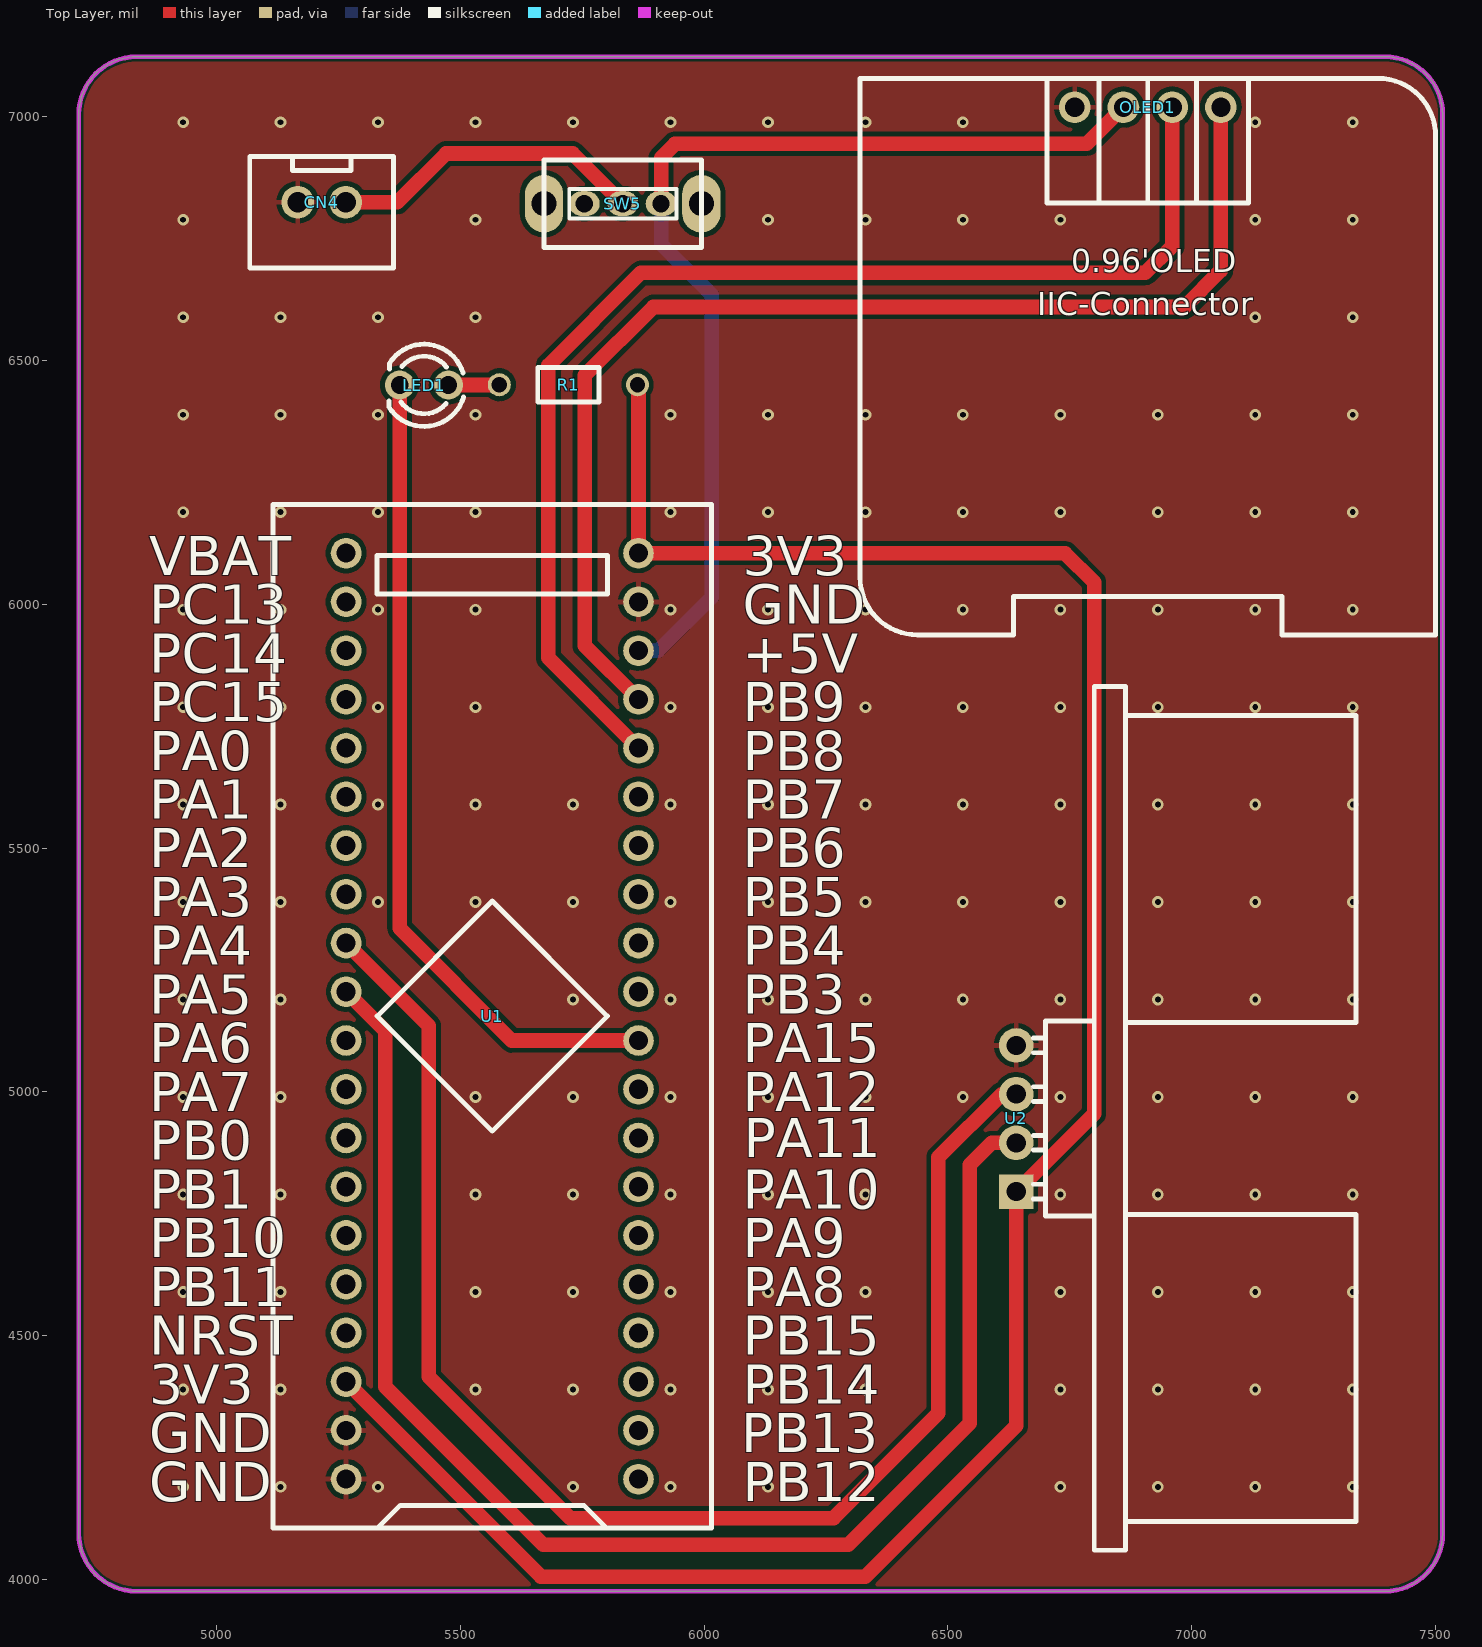
[diagram p0: Top Layer view]
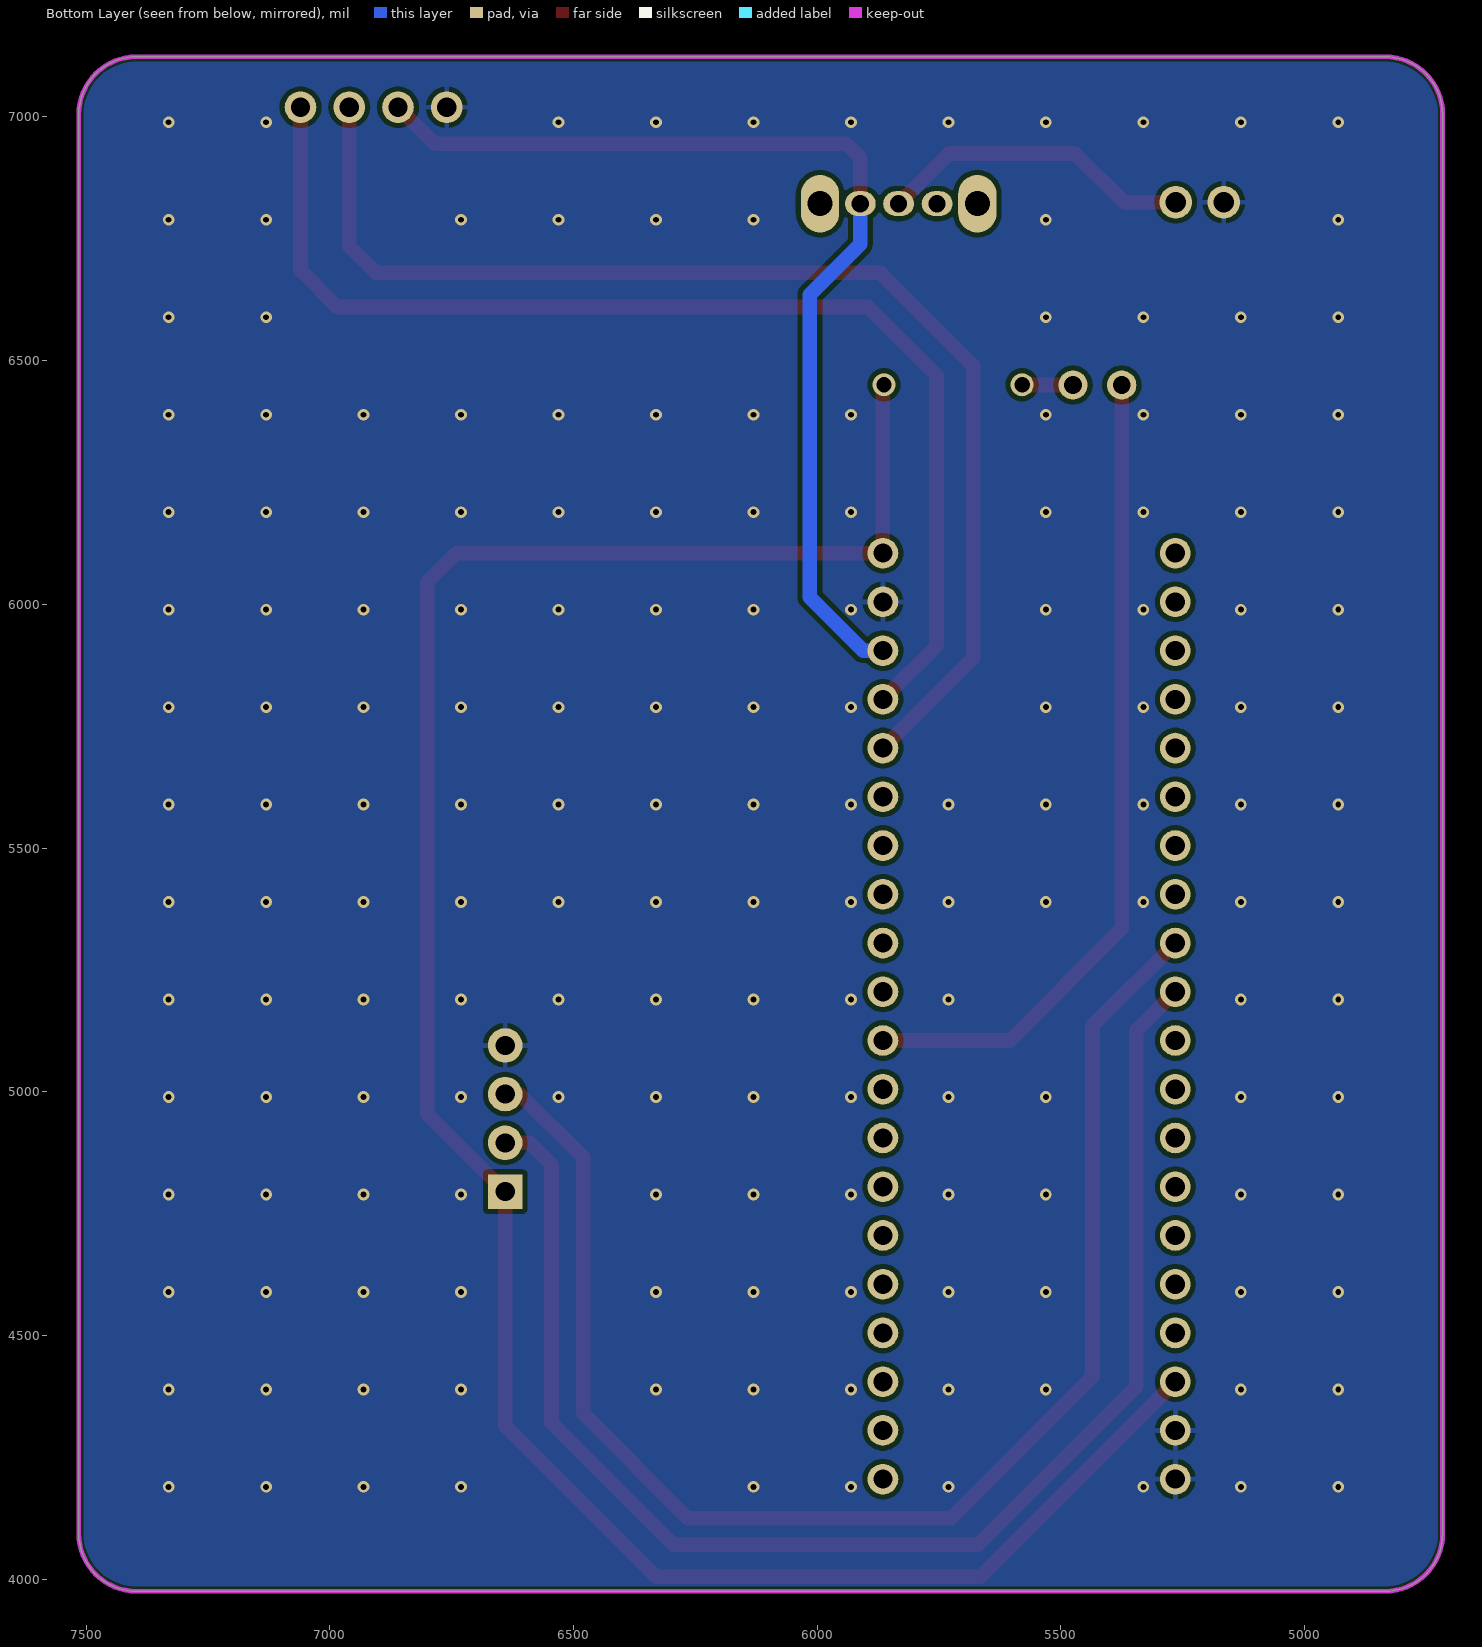
[diagram p1: Bottom Layer view, seen from below]
# Altium PCB MISC89090.pcbdoc
Units mil, origin at the board's own origin, x right, y up, seen from the top; angles counter-clockwise.
Board outline 2798.5 x 3148.5 mil, 2 copper layers (Top Layer, Bottom Layer), stack 62.206 mil thick; 7 components, 39 nets, 59 pads, 165 vias.

## Layer stack, top to bottom
Top Solder Mask Layer: solder mask 0.394, Dk 3.3
Top Layer: signal copper 1.379
Dielectric1: surface 59.449, FR4, Dk 4.5
Bottom Layer: signal copper 1.378
Bottom Solder Mask Layer: solder mask 0.394, Dk 3.3

## Board outline
4834.61,7123.5 ccw(c4834.61,7005.39) 4716.5,7005.39 4716.5,4093.11 ccw(c4834.61,4093.11) 4834.61,3975 7396.89,3975 ccw(c7396.89,4093.11) 7515,4093.11 7515,7005.39 ccw(c7396.89,7005.39) 7396.89,7123.5 4834.61,7123.5

## Design rules (kind name [scope] priority, off if disabled: settings)
BoardOutlineClearance copperThickness2oz_1 [All] p2 off: genericclearance=7.99 ignorepadtopadclearanceinfootprint=FALSE except(0: Arc-SplitContinuation Track-SplitContinuation SMDPad-SplitContinuation THPad-SplitContinuation Via-SplitContinuation Fill-SplitContinuation Region-SplitContinuation Poly-SplitContinuation Text-SplitContinuation Hole-SplitContinuation; 5.98: Arc-CutoutEdge Track-CutoutEdge SMDPad-CutoutEdge THPad-CutoutEdge Via-CutoutEdge Text-CutoutEdge; 6.9: Hole-OutlineEdge Hole-CutoutEdge; 10: Poly-OutlineEdge Poly-CutoutEdge; 11.81: Arc-OutlineEdge Track-OutlineEdge SMDPad-OutlineEdge THPad-OutlineEdge Via-OutlineEdge Fill-OutlineEdge Region-OutlineEdge Text-OutlineEdge Fill-CutoutEdge Region-CutoutEdge)
BoardOutlineClearance Plane_innerPlane_1 [All] p4 off: genericclearance=4.02 ignorepadtopadclearanceinfootprint=FALSE except(0: Arc-SplitContinuation Track-SplitContinuation SMDPad-SplitContinuation THPad-SplitContinuation Via-SplitContinuation Fill-SplitContinuation Region-SplitContinuation Poly-SplitContinuation Text-SplitContinuation Hole-SplitContinuation; 5.98: Arc-CutoutEdge Track-CutoutEdge SMDPad-CutoutEdge THPad-CutoutEdge Via-CutoutEdge Text-CutoutEdge; 6.9: Hole-OutlineEdge Hole-CutoutEdge; 10: Poly-OutlineEdge Poly-CutoutEdge; 11.81: Arc-OutlineEdge Track-OutlineEdge SMDPad-OutlineEdge THPad-OutlineEdge Via-OutlineEdge Fill-OutlineEdge Region-OutlineEdge Text-OutlineEdge Fill-CutoutEdge Region-CutoutEdge)
BoardOutlineClearance Copper_copperRegion_1 [All] p6 off: genericclearance=4.02 ignorepadtopadclearanceinfootprint=FALSE except(0: Arc-SplitContinuation Track-SplitContinuation SMDPad-SplitContinuation THPad-SplitContinuation Via-SplitContinuation Fill-SplitContinuation Region-SplitContinuation Poly-SplitContinuation Text-SplitContinuation Hole-SplitContinuation; 5.98: Arc-CutoutEdge Track-CutoutEdge SMDPad-CutoutEdge THPad-CutoutEdge Via-CutoutEdge Text-CutoutEdge; 6.9: Hole-OutlineEdge Hole-CutoutEdge; 10: Poly-OutlineEdge Poly-CutoutEdge; 11.81: Arc-OutlineEdge Track-OutlineEdge SMDPad-OutlineEdge THPad-OutlineEdge Via-OutlineEdge Fill-OutlineEdge Region-OutlineEdge Text-OutlineEdge Fill-CutoutEdge Region-CutoutEdge)
BoardOutlineClearance copperThickness1oz_1 [All] p8: genericclearance=4.02 ignorepadtopadclearanceinfootprint=FALSE except(0: Arc-SplitContinuation Track-SplitContinuation SMDPad-SplitContinuation THPad-SplitContinuation Via-SplitContinuation Fill-SplitContinuation Region-SplitContinuation Poly-SplitContinuation Text-SplitContinuation Hole-SplitContinuation; 5.98: Arc-CutoutEdge Track-CutoutEdge SMDPad-CutoutEdge THPad-CutoutEdge Via-CutoutEdge Text-CutoutEdge; 6.9: Hole-OutlineEdge Hole-CutoutEdge; 10: Poly-OutlineEdge Poly-CutoutEdge; 11.81: Arc-OutlineEdge Track-OutlineEdge SMDPad-OutlineEdge THPad-OutlineEdge Via-OutlineEdge Fill-OutlineEdge Region-OutlineEdge Text-OutlineEdge Fill-CutoutEdge Region-CutoutEdge)
Clearance copperThickness2oz [All] p1 off: gap=7.99 ignorepadtopadclearanceinfootprint=FALSE except(5.98: SMDPad-Track SMDPad-SMDPad THPad-Track SMDPad-THPad THPad-THPad Track-Via SMDPad-Via THPad-Via Via-Via Fill-SMDPad Region-SMDPad Fill-THPad Region-THPad Fill-Via Region-Via Fill-Fill Fill-Region Region-Region Arc-Track Arc-SMDPad Arc-THPad Arc-Via Fill-Arc Region-Arc Arc-Arc Text-Track SMDPad-Text Text-THPad Text-Via Fill-Text Region-Text Arc-Text Text-Text; 6.9: Hole-Track Hole-SMDPad Hole-THPad Hole-Via Fill-Hole Region-Hole Hole-Arc Hole-Text; 10: Poly-Track Poly-SMDPad Poly-THPad Poly-Via Poly-Fill Poly-Region Poly-Poly Poly-Arc Poly-Text Poly-Hole; 11.81: Fill-Track Region-Track)
Clearance Plane_innerPlane [All] p3 off: gap=4.02 ignorepadtopadclearanceinfootprint=FALSE except(5.98: SMDPad-Track SMDPad-SMDPad THPad-Track SMDPad-THPad THPad-THPad Track-Via SMDPad-Via THPad-Via Via-Via Fill-SMDPad Region-SMDPad Fill-THPad Region-THPad Fill-Via Region-Via Fill-Fill Fill-Region Region-Region Arc-Track Arc-SMDPad Arc-THPad Arc-Via Fill-Arc Region-Arc Arc-Arc Text-Track SMDPad-Text Text-THPad Text-Via Fill-Text Region-Text Arc-Text Text-Text; 6.9: Hole-Track Hole-SMDPad Hole-THPad Hole-Via Fill-Hole Region-Hole Hole-Arc Hole-Text; 10: Poly-Track Poly-SMDPad Poly-THPad Poly-Via Poly-Fill Poly-Region Poly-Poly Poly-Arc Poly-Text Poly-Hole; 11.81: Fill-Track Region-Track)
Clearance Copper_copperRegion [All] p5 off: gap=4.02 ignorepadtopadclearanceinfootprint=FALSE except(5.98: SMDPad-Track SMDPad-SMDPad THPad-Track SMDPad-THPad THPad-THPad Track-Via SMDPad-Via THPad-Via Via-Via Fill-SMDPad Region-SMDPad Fill-THPad Region-THPad Fill-Via Region-Via Fill-Fill Fill-Region Region-Region Arc-Track Arc-SMDPad Arc-THPad Arc-Via Fill-Arc Region-Arc Arc-Arc Text-Track SMDPad-Text Text-THPad Text-Via Fill-Text Region-Text Arc-Text Text-Text; 6.9: Hole-Track Hole-SMDPad Hole-THPad Hole-Via Fill-Hole Region-Hole Hole-Arc Hole-Text; 10: Poly-Track Poly-SMDPad Poly-THPad Poly-Via Poly-Fill Poly-Region Poly-Poly Poly-Arc Poly-Text Poly-Hole; 11.81: Fill-Track Region-Track)
Clearance copperThickness1oz [All] p7: gap=4.02 ignorepadtopadclearanceinfootprint=FALSE except(5.98: SMDPad-Track SMDPad-SMDPad THPad-Track SMDPad-THPad THPad-THPad Track-Via SMDPad-Via THPad-Via Via-Via Fill-SMDPad Region-SMDPad Fill-THPad Region-THPad Fill-Via Region-Via Fill-Fill Fill-Region Region-Region Arc-Track Arc-SMDPad Arc-THPad Arc-Via Fill-Arc Region-Arc Arc-Arc Text-Track SMDPad-Text Text-THPad Text-Via Fill-Text Region-Text Arc-Text Text-Text; 6.9: Hole-Track Hole-SMDPad Hole-THPad Hole-Via Fill-Hole Region-Hole Hole-Arc Hole-Text; 10: Poly-Track Poly-SMDPad Poly-THPad Poly-Via Poly-Fill Poly-Region Poly-Poly Poly-Arc Poly-Text Poly-Hole; 11.81: Fill-Track Region-Track)
DiffPairsRouting differentialPair [All] p1: maxlimit=6 minlimit=6 mostfreqgap=6 toplayer_minwidth=5 toplayer_prefwidth=10 toplayer_maxwidth=100 toplayer_mingap=6 toplayer_prefgap=6 toplayer_maxgap=6 bottomlayer_minwidth=5 bottomlayer_prefwidth=10 bottomlayer_maxwidth=100 bottomlayer_mingap=6 bottomlayer_prefgap=6 bottomlayer_maxgap=6 maxuncoupledlength=10
HoleToHoleClearance otherClearance [All] p1: gap=11.81 allowstackedmicrovias=TRUE
Length netLength [All] p1: minlimit=0 maxlimit=0
PasteMaskExpansion pasteMaskExpansion [All] p1: expansion=0
PlaneConnect innerPlane [All] p1: planeconnectstyle=Relief reliefexpansion=20 reliefentries=4 reliefconductorwidth=10 reliefairgap=10
PolygonConnect copperRegion [All] p1: connectstyle=Relief reliefconductorwidth=10 reliefentries=4 polygonreliefangle="90 Angle" airgapwidth=10 via.connectstyle=Relief via.reliefconductorwidth=10 via.reliefentries=4 via.polygonreliefangle="90 Angle" via.airgapwidth=10
RoutingVias viaSize [All] p1: holewidth=12.01 width=24.02 viastyle="Through Hole" minholewidth=11.81 minwidth=19.68 maxholewidth=248.03 maxwidth=393.7
SolderMaskExpansion solderMaskExpansion [IsVia] p1: expansion=-1000 istentingtop=TRUE
SolderMaskExpansion solderMaskExpansion [All] p2: expansion=2 istentingtop=FALSE
Width copperThickness2oz_2 [All] p1 off: maxlimit=100 minlimit=8 preferedwidth=10
Width copperThickness1oz_2 [All] p2: maxlimit=100 minlimit=5 preferedwidth=10

## Components (designator, comment, footprint, x,y, rotation, side; value= is the part's Value field where it differs from the comment)
CN4 "XH2.54*2P_Through-hole" CONN-TH_2P-P2.50-XH2.54-2P 5215,6825 r0 top
LED1 "" LED_TH-3mm 5425,6450 r180 top
OLED1 "" 0.96OLED_4P 6910,7020 r0 top
R1 "220Ω" Res_1/8W 5721.15,6448.05 r0 top
SW5 "" 拨动开关 5837.9,6822.05 r180 top
U1 "STM32F103C8T6-Card" CONN-TH_L53.3-W22.9_STM32F103C8T6-CARD 5565,5155 r90 top
U2 "HC-SR04" TH_HC-SR04V 6640,4945 r90 top

## Footprints (in the part's own frame and the unit in brackets; to place one, negate y for a bottom-side part, rotate by r counter-clockwise, add the part's x,y. Pads: shape width x height; smd on the part's side, far side on the other; paste and mask are expansions set on the pad)
0.96OLED_4P [mm]
  round 1.65 hole 1 copper offset 0,0: 1(-3.81,-0.001) 2(-1.27,0.002) 3(1.27,0.002) 4(3.81,0.002)
  silkscreen extent -15,-27.5 15,1.5
CONN-TH_2P-P2.50-XH2.54-2P [mm]
  round 1.7 hole 1.05 paste+0 mask+0.05: 1(1.25,0) 2(-1.25,0)
  silkscreen extent -3.75,-3.42 3.75,2.37
CONN-TH_L53.3-W22.9_STM32F103C8T6-CARD [mm]
  round 1.6 hole 1: 1(-24.13,-7.62) 2(-21.59,-7.62) 3(-19.05,-7.62) 4(-16.51,-7.62) 5(-13.97,-7.62) 6(-11.43,-7.62) 7(-8.89,-7.62) 8(-6.35,-7.62) 9(-3.81,-7.62) 10(-1.27,-7.62) 11(1.27,-7.62) 12(3.81,-7.62) 13(6.35,-7.62) 14(8.89,-7.62) 15(11.43,-7.62) 16(13.97,-7.62) 17(16.51,-7.62) 18(19.05,-7.62) 19(21.59,-7.62) 20(24.13,-7.62) 21(24.13,7.62) 22(21.59,7.62) 23(19.05,7.62) 24(16.51,7.62) 25(13.97,7.62) 26(11.43,7.62) 27(8.89,7.62) 28(6.35,7.62) 29(3.81,7.62) 30(1.27,7.62) 31(-1.27,7.62) 32(-3.81,7.62) 33(-6.35,7.62) 34(-8.89,7.62) 35(-11.43,7.62) 36(-13.97,7.62) 37(-16.51,7.62) 38(-19.05,7.62) 39(-21.59,7.62) 40(-24.13,7.62)
  silkscreen extent -26.67,-11.43 26.67,11.43
LED_TH-3mm [mil]
  round 60 hole 36 paste+0 mask+2: 1(-50,0) 2(50,0)
  silkscreen extent -81,-84 72,85
Res_1/8W [mil]
  round 47.2 hole 31.5 paste+0 mask+2: 1(-141.7,2.48) 2(141.7,2.48)
  silkscreen extent -63,-33 63,38
TH_HC-SR04V [mm]
  rect 1.8x1.8 hole 1.001: 1(-3.81,0)
  round 1.8 hole 1.001: 2(-1.27,0) 3(1.27,0) 4(3.81,0)
  silkscreen extent -22.5,-17.7 22.5,-0.89
拨动开关 [mil]
  oval 63x51.2 hole 35.4 paste+0 mask+2: 1(-73.4,0) 2(5,0) 3(84,0)
  oval 78.7x118.1 hole 51.2 paste+0 mask+2: 4(166.7,0) 5(-156.1,0)
  silkscreen extent -156,-90 167,90

## Via types
v1: diameter 24.02, hole 12, Top Layer to Bottom Layer, 165 vias

## Nets (pads, with @x,y where several pads share a name; then routed paths per layer and width w, separated by ;. In a path a pad name is that pad's centre, name@x,y a point inside that pad or via, vN(x,y) a via of type N, cw(c..) or ccw(c..) an arc to the next point about the centre after c; other vN are vias at no path point)
$1N17118: CN4.1 SW5.2 | length 652.7
  Top Layer w30: CN4.1 5370,6825 5470,6925 5729.95,6925 SW5.2
$1N17142: LED1.1 R1.1 | length 104.7
  Top Layer w30: LED1.1 5578.92,6450 R1.1
+5V: OLED1.2 SW5.1 U1.18 | length 2131.5
  Top Layer w30: SW5.1 5911.3,6916.3 5940,6945 6784.95,6945 OLED1.2@6860,7020.05
  Bottom Layer w30: U1.18 5905,5905 6015,6015 6015,6635 5911.3,6738.7 SW5.1
GND: CN4.2 OLED1.1 U1.19 U1.39 U1.40 U2.4
  other v1: 4930.6,4189.1 5130.6,4189.1 5330.6,4189.1 5730.6,4189.1 5930.6,4189.1 6130.6,4189.1 6730.6,4189.1 6930.6,4189.1 7130.6,4189.1 7330.6,4189.1 4930.6,4389.1 5130.6,4389.1 5530.6,4389.1 5730.6,4389.1 5930.6,4389.1 6130.6,4389.1 6330.6,4389.1 6730.6,4389.1 6930.6,4389.1 7130.6,4389.1 7330.6,4389.1 4930.6,4589.1 5130.6,4589.1 5530.6,4589.1 5730.6,4589.1 5930.6,4589.1 6130.6,4589.1 6330.6,4589.1 6730.6,4589.1 6930.6,4589.1 7130.6,4589.1 7330.6,4589.1 4930.6,4789.1 5130.6,4789.1 5530.6,4789.1 5730.6,4789.1 5930.6,4789.1 6130.6,4789.1 6330.6,4789.1 6730.6,4789.1 6930.6,4789.1 7130.6,4789.1 7330.6,4789.1 4930.6,4989.1 5130.6,4989.1 5530.6,4989.1 5730.6,4989.1 5930.6,4989.1 6130.6,4989.1 6330.6,4989.1 6530.6,4989.1 6730.6,4989.1 6930.6,4989.1 7130.6,4989.1 7330.6,4989.1 4930.6,5189.1 5130.6,5189.1 5730.6,5189.1 5930.6,5189.1 6130.6,5189.1 6330.6,5189.1 6530.6,5189.1 6730.6,5189.1 6930.6,5189.1 7130.6,5189.1 7330.6,5189.1 4930.6,5389.1 5130.6,5389.1 5330.6,5389.1 5530.6,5389.1 5730.6,5389.1 5930.6,5389.1 6130.6,5389.1 6330.6,5389.1 6530.6,5389.1 6730.6,5389.1 6930.6,5389.1 7130.6,5389.1 7330.6,5389.1 4930.6,5589.1 5130.6,5589.1 5330.6,5589.1 5530.6,5589.1 5730.6,5589.1 5930.6,5589.1 6130.6,5589.1 6330.6,5589.1 6530.6,5589.1 6730.6,5589.1 6930.6,5589.1 7130.6,5589.1 7330.6,5589.1 4930.6,5789.1 5130.6,5789.1 5330.6,5789.1 5530.6,5789.1 5930.6,5789.1 6130.6,5789.1 6330.6,5789.1 6530.6,5789.1 6730.6,5789.1 6930.6,5789.1 7130.6,5789.1 7330.6,5789.1 4930.6,5989.1 5130.6,5989.1 5330.6,5989.1 5530.6,5989.1 5930.6,5989.1 6130.6,5989.1 6330.6,5989.1 6530.6,5989.1 6730.6,5989.1 6930.6,5989.1 7130.6,5989.1 7330.6,5989.1 4930.6,6189.1 5130.6,6189.1 5330.6,6189.1 5530.6,6189.1 5930.6,6189.1 6130.6,6189.1 6330.6,6189.1 6530.6,6189.1 6730.6,6189.1 6930.6,6189.1 7130.6,6189.1 7330.6,6189.1 4930.6,6389.1 5130.6,6389.1 5330.6,6389.1 5530.6,6389.1 5930.6,6389.1 6130.6,6389.1 6330.6,6389.1 6530.6,6389.1 6730.6,6389.1 6930.6,6389.1 7130.6,6389.1 7330.6,6389.1 4930.6,6589.1 5130.6,6589.1 5330.6,6589.1 5530.6,6589.1 7130.6,6589.1 7330.6,6589.1 4930.6,6789.1 5530.6,6789.1 6130.6,6789.1 6330.6,6789.1 6530.6,6789.1 6730.6,6789.1 7130.6,6789.1 7330.6,6789.1 4930.6,6989.1 5130.6,6989.1 5330.6,6989.1 5530.6,6989.1 5730.6,6989.1 5930.6,6989.1 6130.6,6989.1 6330.6,6989.1 6530.6,6989.1 7130.6,6989.1 7330.6,6989.1
NRST: U1.37
PA0: U1.25
PA1: U1.26
PA2: U1.27
PA3: U1.28
PA4: U1.29 U2.3 | length 2953.4
  Top Layer w30: U1.29 5435,5135 5435,4415 5725,4125 6265,4125 6480,4340 6480,4865 6610,4995 U2.3
PA5: U1.30 U2.2 | length 2925
  Top Layer w30: U1.30 5345,5125 5345,4395 5670,4070 6295,4070 6545,4320 6545,4850 6590,4895 U2.2
PA6: U1.31
PA7: U1.32
PA8: U1.5
PA9: U1.6
PA10: U1.7
PA11: U1.8
PA12: U1.9
PA15: LED1.2 U1.10 | length 1700.3
  Top Layer w30: LED1.2 5375,5335 5605,5105 U1.10
PB0: U1.33
PB1: U1.34
PB3: U1.11
PB4: U1.12
PB5: U1.13
PB6: U1.14
PB7: U1.15
PB8: OLED1.3 U1.16 | length 2528.2
  Top Layer w30: U1.16 5680,5890 5680,6490 5870,6680 6905,6680 6960,6735 OLED1.3@6960,7020.05
PB9: OLED1.4 U1.17 | length 2439.7
  Top Layer w30: U1.17 5755,5915 5755,6470 5895,6610 6985,6610 7060,6685 OLED1.4@7060,7020.05
PB10: U1.35
PB11: U1.36
PB12: U1.1
PB13: U1.2
PB14: U1.3
PB15: U1.4
PC13: U1.22
PC14: U1.23
PC15: U1.24
VBAT: U1.21
VCC: R1.2 U1.20 U1.38 U2.1 | length 4771.6
  Top Layer w30: U1.38 5665,4005 6330,4005 6640,4315 U2.1 6800,4955 6800,6045 6740,6105 U1.20 5865,6448.38 R1.2
pads on no net: SW5.3 SW5.4 SW5.5

## Polygon pours and split planes (outlines as drawn)
GND on Bottom Layer (solid, remove dead copper, pour order 2): 3525,7245 3525,3080 7700,3080 7700,7245
GND on Top Layer (solid, remove dead copper, pour order 2): 3000,7415 3000,3000 7930,3000 7930,7415

## Keep-outs
Board Outline Layer:
  the board outline again, w10

## Silkscreen, mask and mechanical layers (free items; w line width, h text height)
Top Silkscreen Layer:
  text "VBAT" at 4860.95,6060 h80
  text "3V3" at 6079.16,6060 h80
  text "PC13" at 4860.95,5960 h80
  text "GND" at 6079.16,5960 h80
  text "PC14" at 4860.95,5860 h80
  text "+5V" at 6079.16,5860 h80
  text "PC15" at 4860.95,5760 h80
  text "PB9" at 6079.16,5760 h80
  text "PA0" at 4860.95,5660 h80
  text "PB8" at 6079.16,5660 h80
  text "PA1" at 4860.95,5560 h80
  text "PB7" at 6079.16,5560 h80
  text "PA2" at 4860.95,5460 h80
  text "PB6" at 6079.16,5460 h80
  text "PA3" at 4860.95,5360 h80
  text "PB5" at 6079.16,5360 h80
  text "PA4" at 4860.95,5260 h80
  text "PB4" at 6079.16,5260 h80
  text "PA5" at 4860.95,5160 h80
  text "PB3" at 6079.16,5160 h80
  text "PA6" at 4860.95,5060 h80
  text "PA15" at 6079.16,5060 h80
  text "PA7" at 4860.95,4960 h80
  text "PA12" at 6079.16,4960 h80
  text "PA11" at 6080.95,4865 h80
  text "PB0" at 4860.95,4860 h80
  text "PB1" at 4860.95,4760 h80
  text "PA10" at 6079.16,4760 h80
  text "PB10" at 4860.95,4660 h80
  text "PA9" at 6079.16,4660 h80
  text "PB11" at 4860.95,4560 h80
  text "PA8" at 6079.16,4560 h80
  text "NRST" at 4860.95,4460 h80
  text "PB15" at 6079.16,4460 h80
  text "3V3" at 4860.95,4360 h80
  text "PB14" at 6079.16,4360 h80
  text "GND" at 4860.95,4260 h80
  text "PB13" at 6075.95,4260 h80
  text "GND" at 4860.95,4160 h80
  text "PB12" at 6079.16,4160 h80